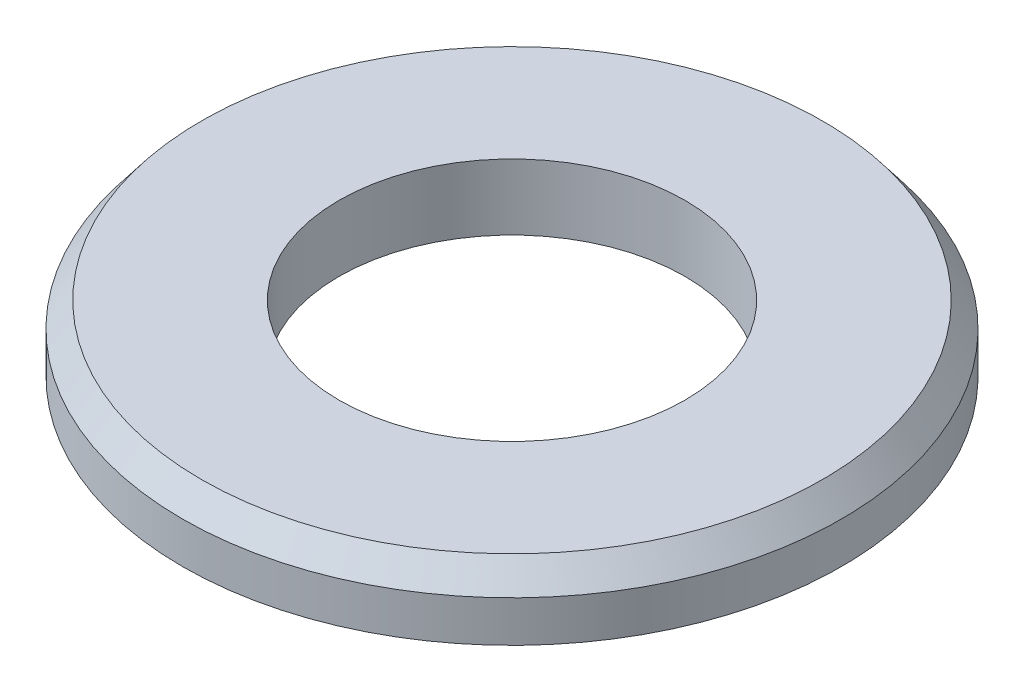
SolidWorks part; units mm, degrees
material "合金钢"
ref_plane "Front Plane" through (0, 0, 0) normal (0, 0, 1) x (1, 0, 0)
ref_plane "Top Plane" through (0, 0, 0) normal (0, 1, 0) x (1, 0, 0)
ref_plane "Right Plane" through (0, 0, 0) normal (1, 0, 0) x (0, 0, -1)
sketch "Sketch1" plane through (0, 0, 0) normal (0, 1, 0) x (1, 0, 0)
  circle A0 centre (0, 0) radius 5.25
  circle A1 centre (0, 0) radius 10
extrude "Boss-Extrude1" add sketch "Sketch1" along normal blind 2
chamfer "Chamfer1" distance 0.75 angle 37.5 1 edges at (0, 2, 10)
